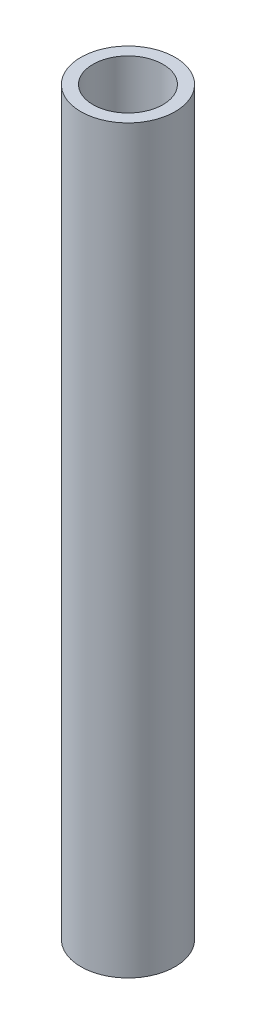
SolidWorks part; units mm, degrees
ref_plane "前基準面" through (0, 0, 0) normal (0, 0, 1) x (1, 0, 0)
ref_plane "上基準面" through (0, 0, 0) normal (0, 1, 0) x (1, 0, 0)
ref_plane "右基準面" through (0, 0, 0) normal (1, 0, 0) x (0, 0, -1)
sketch "草图1" plane through (0, 0, 0) normal (0, 1, 0) x (1, 0, 0)
  circle A0 centre (0, 0) radius 17.5
  dimension "D1" = 35
extrude "凸台-拉伸1" add sketch "草图1" along normal blind 275
shell "抽壳1" thickness 4.5
